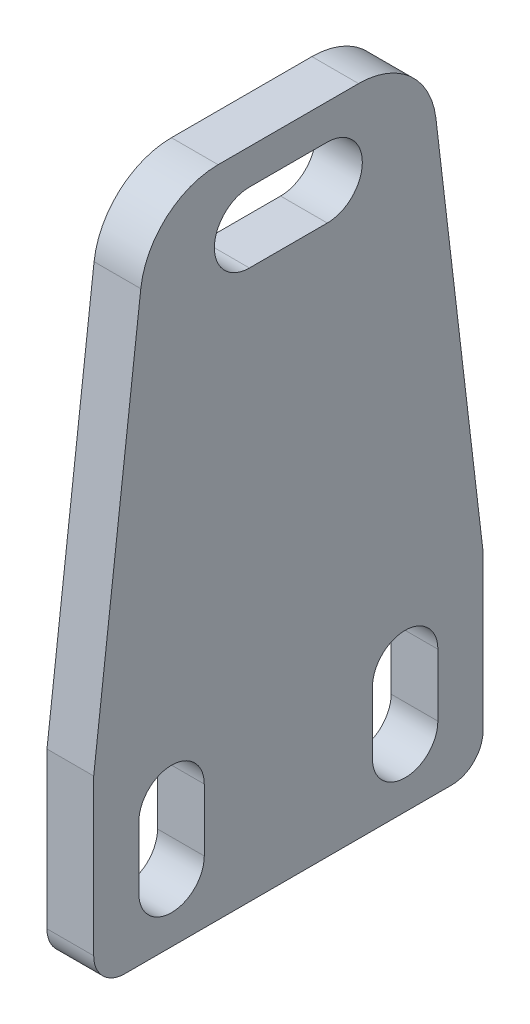
from build123d import *

# Parameters (mm, degrees)
EXTRUDE_1_DEPTH             = 3
EXTRUDE_2_DEPTH             = 3
FILLET_1_R                  = 2
CUT_EXTRUDE_1_DEPTH         = 3
FILLET_2_R                  = 2
HOLE_WIZARD_4_3_4_3_1_D     = 4.3
HOLE_WIZARD_4_3_4_3_1_DEPTH = 10.1
HOLE_WIZARD_4_3_4_3_1_TIP   = 1.291850331
SKETCH_7_W                  = 24.449376322
SKETCH_7_H                  = 27.885292322
CUT_EXTRUDE_2_DEPTH         = 10
CUT_EXTRUDE_3_DEPTH         = 10
FILLET_3_R                  = 5


with BuildPart() as part:
    # 草图1 → 凸台-拉伸1 (new body)
    with BuildSketch(Plane(origin=(0, 0, 0), x_dir=(0, 0, -1), z_dir=(1, 0, 0))):
        Polygon((-12.5, 6), (-6, 6), (-6, 61), (6, 61), (6, 6), (12.5, 6), (12.5, -6), (-12.5, -6), align=None)
    extrude(amount=EXTRUDE_1_DEPTH)

    # 草图2 → 凸台-拉伸2 (add)
    with BuildSketch(Plane.ZY):
        Polygon((-6, 61), (-12.5, 6), (12.5, 6), (6, 61), align=None)
    extrude(amount=-EXTRUDE_2_DEPTH)

    # 圆角1
    fillet_1_edges = [part.edges().sort_by_distance(p)[0] for p in [
        (1.5, 61, 6),
        (1.5, 61, -6),
    ]]
    fillet(fillet_1_edges, radius=FILLET_1_R)

    # 草图3 → 切除-拉伸1 (cut)
    with BuildSketch(Plane.ZY):
        with BuildLine():
            Line((-5.4, 2), (-5.4, -2))
            ThreePointArc((-5.4, -2), (-7.5, -4.1), (-9.6, -2))
            Line((-9.6, -2), (-9.6, 2))
            ThreePointArc((-9.6, 2), (-7.5, 4.1), (-5.4, 2))
        make_face()
        with BuildLine():
            Line((5.4, 2), (5.4, -2))
            ThreePointArc((5.4, -2), (7.5, -4.1), (9.6, -2))
            Line((9.6, -2), (9.6, 2))
            ThreePointArc((9.6, 2), (7.5, 4.1), (5.4, 2))
        make_face()
    extrude(amount=-CUT_EXTRUDE_1_DEPTH, mode=Mode.SUBTRACT)

    # 圆角2
    fillet_2_edges = [part.edges().sort_by_distance(p)[0] for p in [
        (1.5, -6, -12.5),
        (1.5, -6, 12.5),
    ]]
    fillet(fillet_2_edges, radius=FILLET_2_R)

    # Ø4.3 (4.3) 直径孔1
    with Locations(Plane.ZY):
        with Locations((0, 56), (0, 41)):
            Hole(HOLE_WIZARD_4_3_4_3_1_D / 2, depth=HOLE_WIZARD_4_3_4_3_1_DEPTH)
            with Locations((0, 0, -(HOLE_WIZARD_4_3_4_3_1_DEPTH + HOLE_WIZARD_4_3_4_3_1_TIP / 2))):  # 118° drill point
                Cone(0, HOLE_WIZARD_4_3_4_3_1_D / 2, HOLE_WIZARD_4_3_4_3_1_TIP, mode=Mode.SUBTRACT)

    # 草图7 → 切除-拉伸2 (cut)
    with BuildSketch(Plane(origin=(3, 0, 0), x_dir=(0, 0, -1), z_dir=(1, 0, 0))):
        with Locations((-1.251346032, 49.942646161)):
            Rectangle(SKETCH_7_W, SKETCH_7_H)
    extrude(amount=-CUT_EXTRUDE_2_DEPTH, mode=Mode.SUBTRACT)

    # 草图8 → 切除-拉伸3 (cut)
    with BuildSketch(Plane.ZY):
        with BuildLine():
            Line((-2.5, 33.75), (2.5, 33.75))
            ThreePointArc((2.5, 33.75), (4.75, 31.5), (2.5, 29.25))
            Line((2.5, 29.25), (-2.5, 29.25))
            ThreePointArc((-2.5, 29.25), (-4.75, 31.5), (-2.5, 33.75))
        make_face()
    extrude(amount=-CUT_EXTRUDE_3_DEPTH, mode=Mode.SUBTRACT)

    # 圆角3
    fillet_3_edges = [part.edges().sort_by_distance(p)[0] for p in [
        (1.5, 36, 8.954545455),
        (1.5, 36, -8.954545455),
    ]]
    fillet(fillet_3_edges, radius=FILLET_3_R)


solid = part.part
